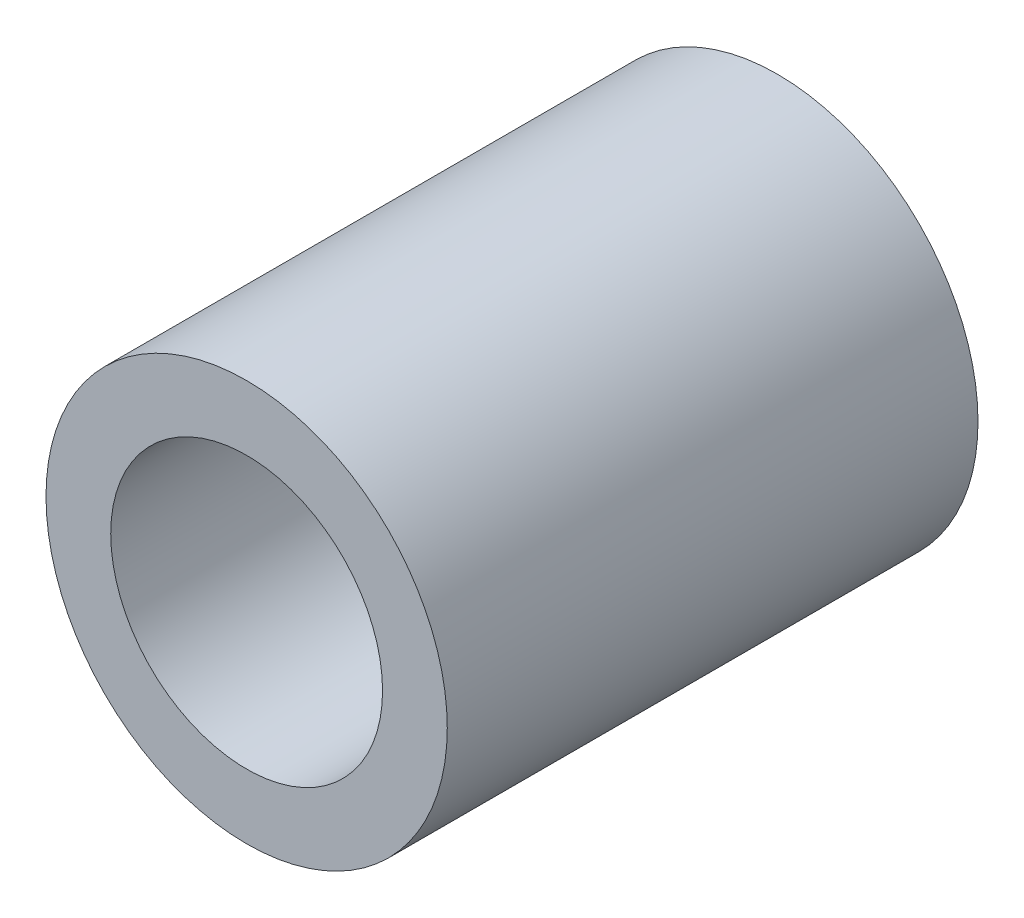
from build123d import *

# Parameters (mm, degrees)
SKETCH1_R           = 15.5
SKETCH1_R_2         = 10.5
BOSS_EXTRUDE1_DEPTH = 41


with BuildPart() as part:
    # Sketch1 → Boss-Extrude1 (new body)
    with BuildSketch(Plane.XY):
        Circle(SKETCH1_R)
        Circle(SKETCH1_R_2, mode=Mode.SUBTRACT)
    extrude(amount=BOSS_EXTRUDE1_DEPTH)


solid = part.part
